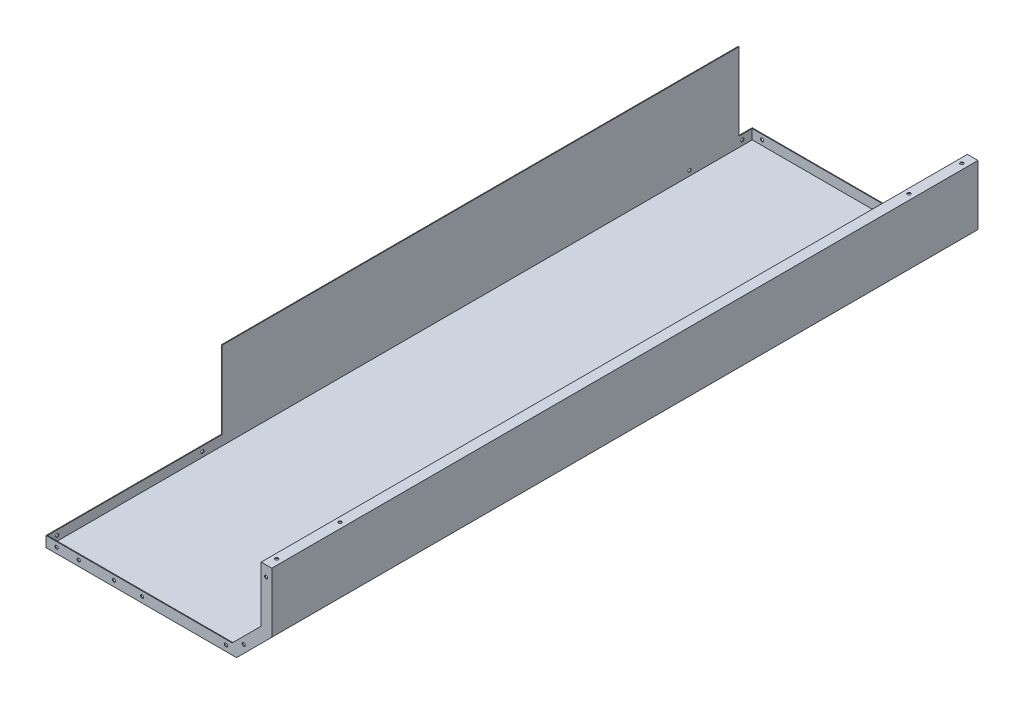
SolidWorks part; units mm, degrees
ref_plane "前视基准面" through (0, 0, 0) normal (0, 0, 1) x (1, 0, 0)
ref_plane "上视基准面" through (0, 0, 0) normal (0, 1, 0) x (1, 0, 0)
ref_plane "右视基准面" through (0, 0, 0) normal (1, 0, 0) x (0, 0, -1)
sketch "草图1" plane through (0, 0, 0) normal (0, 0, 1) x (1, 0, 0)
  line L0 (0, 0) -> (541, 0)
  line L1 (641, 100) -> (641, 270)
  line L2 (541, 0) -> (641, 100)
  point P1 (641, 0)
  dimension "D1" = 641
  dimension "D2" = 270
extrude "拉伸-薄壁1" add sketch "草图1" along normal blind 2005 thin thin type one direction reverse wall 2
sketch "草图4" plane through (639, 0, 0) normal (-1, 0, 0) x (0, 0, 1)
  line L0 (0, 100.8284) -> (0, 270)
  line L1 (0, 270) -> (2005, 270)
  line L2 (2005, 270) -> (2005, 100.8284)
  line L3 (2, 100.8284) -> (2, 268)
  line L4 (2, 268) -> (2003, 268)
  line L5 (2003, 268) -> (2003, 100.8284)
  line L6 (2003, 100.8284) -> (2005, 100.8284)
  line L7 (0, 100.8284) -> (2, 100.8284)
  dimension "D1" = 2
extrude "凸台-拉伸1" add sketch "草图4" along normal blind 28
sketch "草图5" plane through (269.0858, -269.0858, 0) normal (-0.7071, 0.7071, 0) x (0, 0, 1)
  line L0 (0, 523.1377) -> (0, 383.3732)
  line L1 (2005, 523.1377) -> (2005, 383.3732)
  line L2 (2003, 523.1377) -> (2003, 383.3732)
  line L3 (2, 523.1377) -> (2, 383.3732)
  line L4 (0, 523.1377) -> (2, 523.1377)
  line L5 (0, 383.3732) -> (2, 383.3732)
  line L6 (2003, 523.1377) -> (2005, 523.1377)
  line L7 (2003, 383.3732) -> (2005, 383.3732)
  dimension "D1" = 2
  dimension "D2" = 2
extrude "凸台-拉伸2" add sketch "草图5" along normal blind 28
sketch "草图6" plane through (0, 2, 0) normal (0, 1, 0) x (1, 0, 0)
  line L1 (0, 0) -> (540.1716, 0)
  line L2 (0, 0) -> (0, -2)
  line L3 (0, -2) -> (540.1716, -2)
  line L4 (540.1716, 0) -> (540.1716, -2)
  line L5 (0, -2005) -> (540.1716, -2005)
  line L6 (0, -2005) -> (0, -2003)
  line L7 (0, -2003) -> (540.1716, -2003)
  line L8 (540.1716, -2005) -> (540.1716, -2003)
extrude "凸台-拉伸3" add sketch "草图6" along normal blind 28
sketch "草图7" plane through (0, 2, 0) normal (0, 1, 0) x (1, 0, 0)
  line L0 (0, -2005) -> (528.5736, -2005) construction
  line L1 (0, 0) -> (2, 0)
  line L2 (0, 0) -> (0, -2005)
  line L3 (0, -2005) -> (2, -2005)
  line L4 (2, 0) -> (2, -2005)
  dimension "D1" = 2
extrude "凸台-拉伸4" add sketch "草图7" along normal blind 28
sketch "草图8" plane through (0, 30, 0) normal (0, 1, 0) x (1, 0, 0)
  line L0 (0, 0) -> (0, -2005) construction
  line L1 (0, -40) -> (2, -40)
  line L2 (0, -40) -> (0, -1507)
  line L3 (0, -1507) -> (2, -1507)
  line L4 (2, -40) -> (2, -1507)
  line L5 (2, -2003) -> (2, -2) construction
  line L7 (528.5736, 0) -> (0, 0) construction
  dimension "D1" = 1467
  dimension "D2" = 40
extrude "凸台-拉伸5" add sketch "草图8" along normal blind 220
sketch "草图9" plane through (0, 0, 2) normal (0, 0, 1) x (1, 0, 0)
  line L0 (2, 16) -> (569.4303, 16) construction
  line L1 (2, 30) -> (2, 2) construction
  line L2 (625, 268) -> (625, 12) construction
  line L3 (611, 268) -> (639, 268) construction
  line L4 (0, 0) -> (0, 30) construction
  line L5 (611, 270) -> (641, 270) construction
  circle A0 centre (625, 240) radius 4.5
  circle A1 centre (30, 16) radius 4.5
  circle A2 centre (431, 16) radius 4.5
  circle A3 centre (625, 140) radius 4.5
  dimension "D1" = 9
  dimension "D2" = 9
  dimension "D3" = 9
  dimension "D4" = 9
  dimension "D5" = 30
  dimension "D6" = 401
  dimension "D7" = 30
  dimension "D8" = 100
extrude "切除-拉伸1" cut sketch "草图9" against normal blind 10
sketch "草图11" plane through (0, 268, 0) normal (0, -1, 0) x (1, 0, 0)
  line L0 (625, 208.9272) -> (625, -14.4231) construction
  line L1 (611, 2) -> (611, 2003) construction
  line L2 (541, 0) -> (641, 0) construction
  circle A0 centre (625, 30) radius 4.5
  circle A1 centre (625, 180) radius 4.5
  dimension "D2" = 9
  dimension "D3" = 9
  dimension "D4" = 30
  dimension "D5" = 150
  dimension "D1" = 14
extrude "切除-拉伸2" cut sketch "草图11" against normal blind 10
sketch "草图12" plane through (2, 0, 0) normal (1, 0, 0) x (0, 0, -1)
  line L0 (-2, 16) -> (-728.8525, 16) construction
  line L1 (-2, 2) -> (-2, 30) construction
  line L2 (0, 0) -> (0, 30) construction
  circle A0 centre (-30, 16) radius 4.5
  circle A1 centre (-180, 16) radius 4.5
  dimension "D1" = 9
  dimension "D2" = 9
  dimension "D3" = 30
  dimension "D4" = 150
extrude "切除-拉伸3" cut sketch "草图12" against normal blind 116
sketch "草图13" plane through (0, 268, 0) normal (0, -1, 0) x (1, 0, 0)
  line L0 (625, 2003) -> (625, 1903.1768) construction
  line L1 (611, 2003) -> (639, 2003) construction
  line L2 (611, 2005) -> (641, 2005) construction
  circle A0 centre (625, 1975) radius 4.5
  circle A1 centre (625, 1795) radius 4.5
  dimension "D1" = 9
  dimension "D2" = 9
  dimension "D3" = 30
  dimension "D4" = 180
extrude "切除-拉伸4" cut sketch "草图13" against normal blind 63
sketch "草图14" plane through (2, 0, 0) normal (1, 0, 0) x (0, 0, -1)
  line L0 (-2003, 16) -> (-1123, 16) construction
  line L1 (-2003, 30) -> (-2003, 2) construction
  line L2 (-2005, 0) -> (-2005, 30) construction
  circle A0 centre (-1975, 16) radius 4.5
  circle A1 centre (-1563, 16) radius 4.5
  dimension "D1" = 412
  dimension "D2" = 30
  dimension "D3" = 9
  dimension "D4" = 9
extrude "切除-拉伸5" cut sketch "草图14" against normal blind 72
sketch "草图15" plane through (0, 0, 2003) normal (0, 0, -1) x (-1, 0, 0)
  line L0 (-625, 268) -> (-625, 18.9635) construction
  line L1 (-611, 268) -> (-639, 268) construction
  line L2 (-528.3605, 9.9879) -> (-625, 106.6274) construction
  line L3 (-611, 112.4264) -> (-528.5736, 30) construction
  line L4 (-611, 270) -> (-641, 270) construction
  line L5 (-2, 16) -> (-690.7378, 16) construction
  line L6 (-2, 30) -> (-2, 2) construction
  line L7 (0, 0) -> (0, 30) construction
  circle A0 centre (-625, 240) radius 4.5
  circle A1 centre (-561.3604, 42.9878) radius 4.5
  circle A2 centre (-30, 16) radius 4.5
  circle A3 centre (-511, 16) radius 4.5
  circle A4 centre (-273, 16) radius 4.5
  circle A5 centre (-193, 16) radius 4.5
  circle A6 centre (-93, 16) radius 4.5
  dimension "D2" = 9
  dimension "D3" = 9
  dimension "D4" = 90
  dimension "D5" = 30
  dimension "D6" = 9
  dimension "D7" = 30
  dimension "D8" = 9
  dimension "D9" = 481
  dimension "D10" = 9
  dimension "D12" = 9
  dimension "D13" = 9
  dimension "D14" = 80
  dimension "D15" = 100
  dimension "D1" = 14
  dimension "D11" = 238
extrude "切除-拉伸6" cut sketch "草图15" against normal up to vertex (2 mm away)
